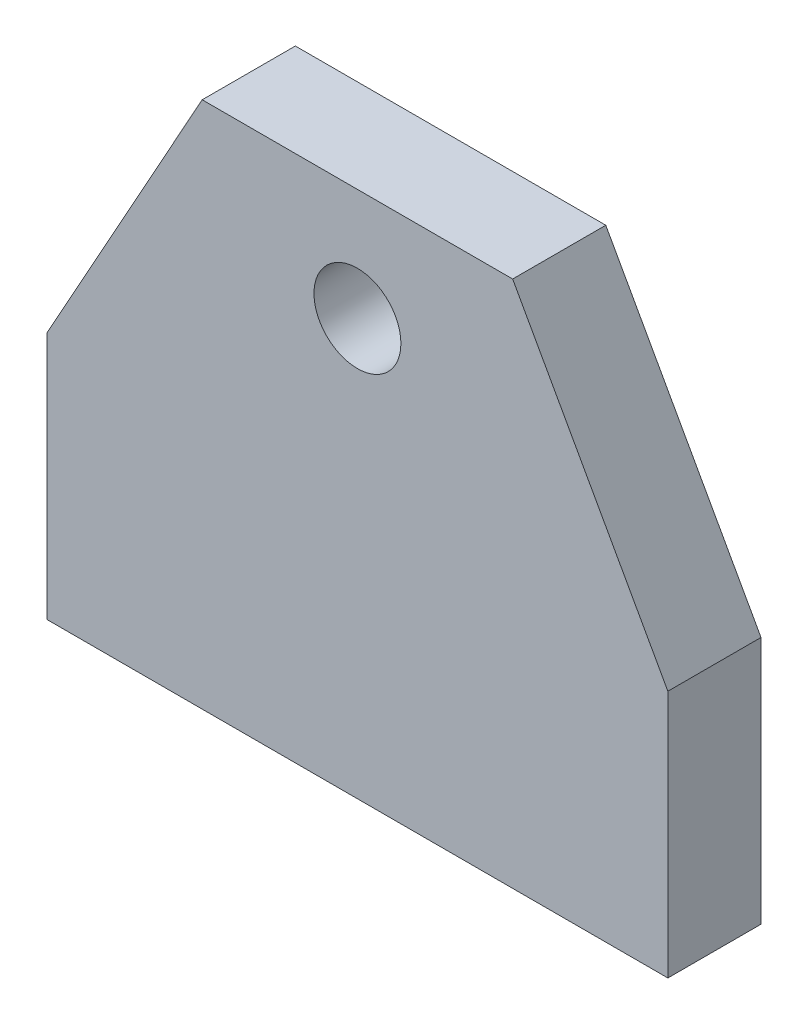
from build123d import *

# Parameters (mm, degrees)
BOSS_EXTRUDE1_DEPTH = 7.5
M16_TAPPED_HOLE1_D  = 14


with BuildPart() as part:
    # Sketch1 → Boss-Extrude1 (new, symmetric)
    with BuildSketch(Plane.XY):
        Polygon((-50, 0), (50, 0), (50, 40), (25, 85), (-25, 85), (-50, 40), align=None)
    extrude(amount=BOSS_EXTRUDE1_DEPTH, both=True)

    # M16 Tapped Hole1 (through all)
    with Locations(Plane(origin=(0, 67, 7.5), x_dir=(1, 0, 0), z_dir=(0, 0, 1))):
        with Locations((0, 0)):
            Hole(M16_TAPPED_HOLE1_D / 2)


solid = part.part
